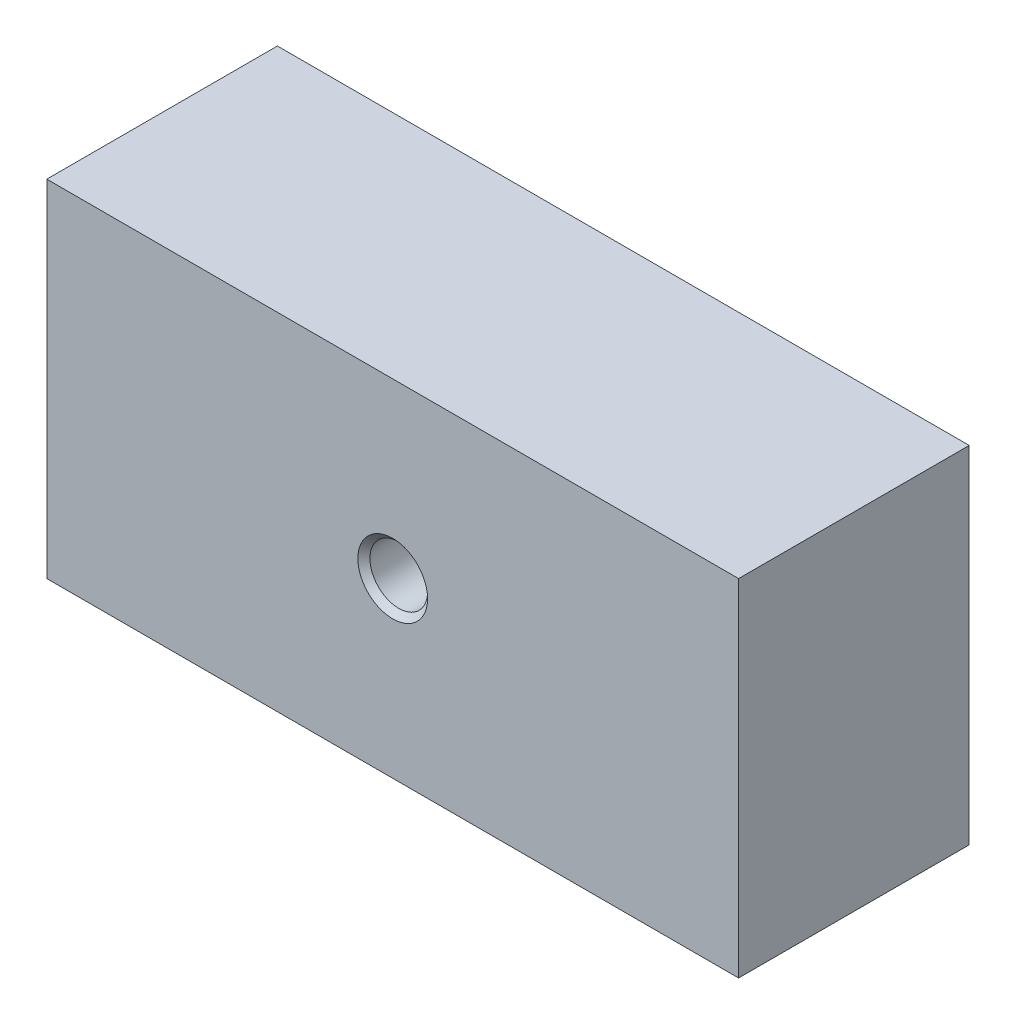
SolidWorks part; units mm, degrees
ref_plane "Front Plane" through (0, 0, 0) normal (0, 0, 1) x (1, 0, 0)
ref_plane "Top Plane" through (0, 0, 0) normal (0, 1, 0) x (1, 0, 0)
ref_plane "Right Plane" through (0, 0, 0) normal (1, 0, 0) x (0, 0, -1)
sketch "Sketch1" plane through (0, 0, 0) normal (0, 0, 1) x (1, 0, 0)
  line L0 (748, 60) -> (739, 60) construction
  line L1 (690, 30) -> (750, 30)
  line L2 (690, 30) -> (690, 60)
  line L3 (690, 60) -> (750, 60)
  line L4 (750, 30) -> (750, 60)
  line L5 (750, 50) -> (750, 58) construction
extrude "Boss-Extrude1" add sketch "Sketch1" along normal blind 20
sketch "Sketch2" plane through (0, 0, 20) normal (0, 0, 1) x (1, 0, 0)
  line L0 (720, 60) -> (720, 45) construction
  line L1 (750, 60) -> (690, 60) construction
  line L2 (720, 45) -> (750, 45) construction
  line L3 (750, 30) -> (750, 60) construction
hole_wizard "M6 Tapped Hole1" positions "Sketch3" profile "Sketch4" tap size "M6" standard "GB"
sketch "Sketch3" plane through (0, 0, 20) normal (0, 0, 1) x (1, 0, 0)
  point P0 (720, 45)
sketch "Sketch4" plane through (720, 45, 20) normal (1, 0, 0) x (0, -1, 0)
  line L0 (0, 0) -> (0, 16.5022)
  line L1 (0, 16.5022) -> (2.5, 15)
  line L2 (2.5, 15) -> (2.5, 0.525)
  line L3 (2.5, 0.525) -> (3.025, 0)
  line L5 (3.025, 0) -> (0, 0)
  line L6 (-2.5, 0.525) -> (-3.025, 0) construction
  line L10 (0, 16.5022) -> (-2.5, 15) construction
  line L11 (0, -6.35) -> (0, 107.95) construction
  dimension "螺纹孔钻头直径" = 5
  dimension "螺纹孔钻头深度" = 15
  dimension "近端锥形沉头孔直径" = 6.05
  dimension "近端锥形沉头孔角度" = 90
  dimension "导头角度" = 118
cosmetic thread "Cosmetic Thread1"
